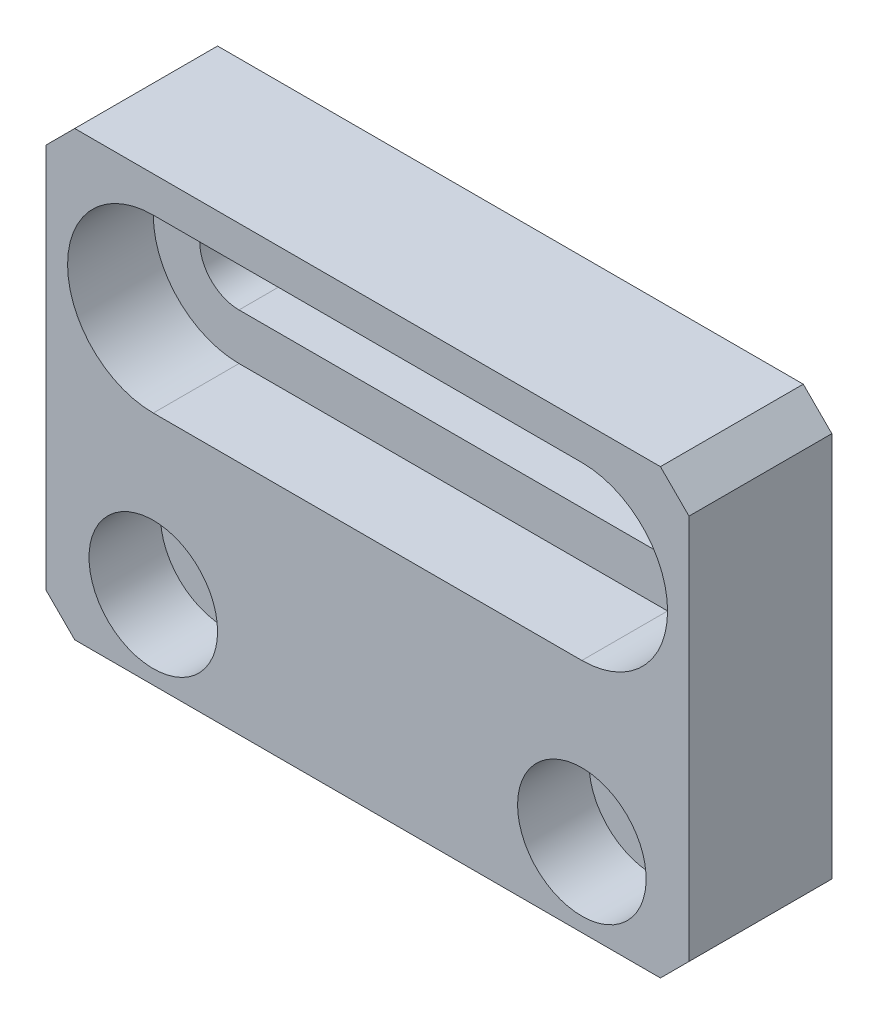
SolidWorks part; units mm, degrees
ref_plane "Front Plane" through (0, 0, 0) normal (0, 0, 1) x (1, 0, 0)
ref_plane "Top Plane" through (0, 0, 0) normal (0, 1, 0) x (1, 0, 0)
ref_plane "Right Plane" through (0, 0, 0) normal (1, 0, 0) x (0, 0, -1)
sketch "Sketch1" plane through (0, 0, 0) normal (0, 0, 1) x (1, 0, 0)
  line L1 (-22.5, 15.5) -> (22.5, 15.5)
  line L2 (-22.5, 15.5) -> (-22.5, -15.5)
  line L3 (-22.5, -15.5) -> (22.5, -15.5)
  line L4 (22.5, 15.5) -> (22.5, -15.5)
  line L5 (-22.5, 15.5) -> (22.5, -15.5) construction
  line L6 (-22.5, -15.5) -> (22.5, 15.5) construction
  point P0 (0, 0)
  dimension "D1" = 31
  dimension "D2" = 45
extrude "Boss-Extrude1" add sketch "Sketch1" along normal blind 10
sketch "Sketch2" plane through (0, 0, 10) normal (0, 0, 1) x (1, 0, 0)
  line L0 (0, 0) -> (0, 50000) construction
  line L1 (-15, 7) -> (15, 7) construction
  line L2 (-15, 9.75) -> (15, 9.75)
  line L3 (-15, 4.25) -> (15, 4.25)
  line L4 (-22.5, -15.5) -> (22.5, -15.5) construction
  arc A0 (-15, 9.75) -> (-15, 4.25) centre (-15, 7) ccw
  arc A1 (15, 4.25) -> (15, 9.75) centre (15, 7) ccw
  point P5 (0, 7)
  dimension "D1" = 5.5
  dimension "D2" = 30
  dimension "D3" = 22.5
extrude "Cut-Extrude1" cut sketch "Sketch2" against normal blind 13
sketch "Sketch3" plane through (0, 0, 10) normal (0, 0, 1) x (1, 0, 0)
  line L0 (0, 0) -> (0, -50000) construction
  line L1 (-22.5, -15.5) -> (22.5, -15.5) construction
  circle A0 centre (-15, -10) radius 4.5
  circle A1 centre (15, -10) radius 4.5
  dimension "D1" = 30
  dimension "D2" = 9
  dimension "D3" = 5.5
extrude "Cut-Extrude2" cut sketch "Sketch3" against normal blind 5
sketch "Sketch4" plane through (0, 0, 10) normal (0, 0, 1) x (1, 0, 0)
  circle A0 centre (-15, -10) radius 2.25
  circle A1 centre (15, -10) radius 2.25
  dimension "D1" = 4.5
extrude "Cut-Extrude3" cut sketch "Sketch4" against normal blind 14
chamfer "Chamfer1" distance 2 angle 45 4 edges at (22.5, 15.5, 5) (-22.5, 15.5, 5) (22.5, -15.5, 5) (-22.5, -15.5, 5)
sketch "Sketch5" plane through (0, 0, 10) normal (0, 0, 1) x (1, 0, 0)
  line L0 (-15, 7) -> (15, 7) construction
  line L1 (-15, 13) -> (15, 13)
  line L2 (-15, 1) -> (15, 1)
  arc A0 (-15, 13) -> (-15, 1) centre (-15, 7) ccw
  arc A1 (15, 1) -> (15, 13) centre (15, 7) ccw
  point P4 (0, 7)
  dimension "D1" = 12
extrude "Cut-Extrude4" cut sketch "Sketch5" against normal blind 6
